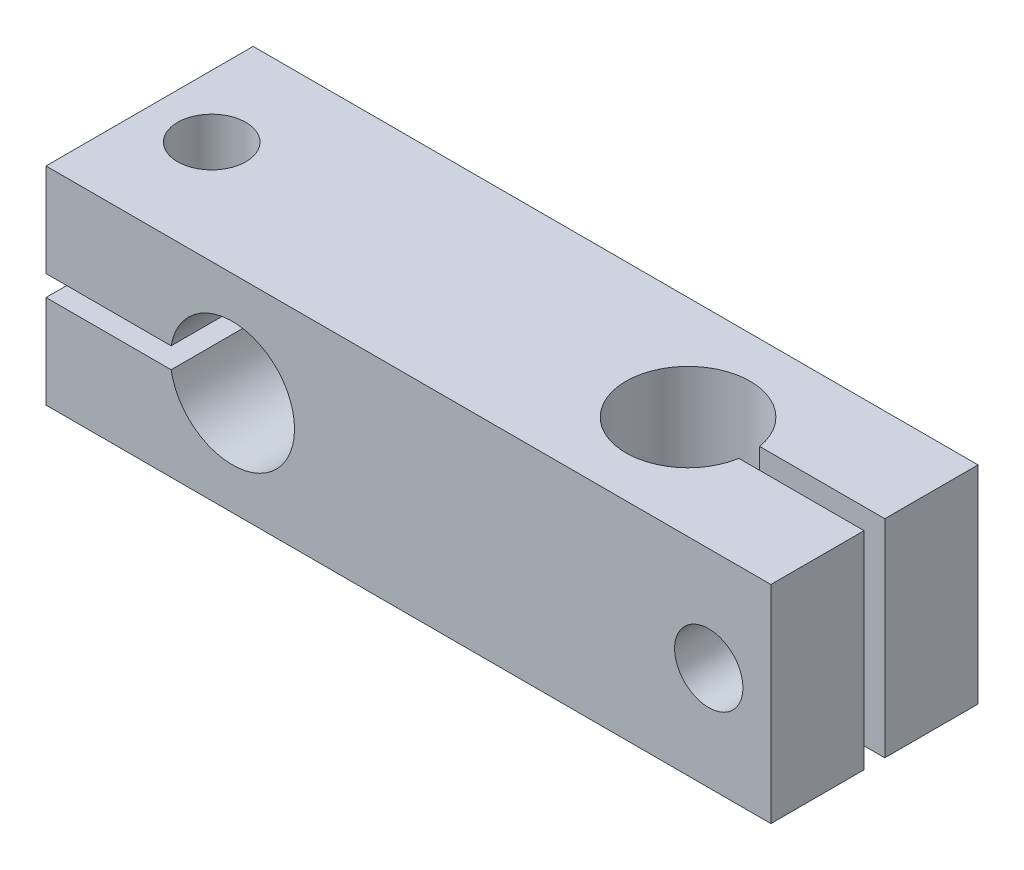
SolidWorks part; units mm, degrees
material "Q235-A"
ref_plane "Front Plane" through (0, 0, 0) normal (0, 0, 1) x (1, 0, 0)
ref_plane "Top Plane" through (0, 0, 0) normal (0, 1, 0) x (1, 0, 0)
ref_plane "Right Plane" through (0, 0, 0) normal (1, 0, 0) x (0, 0, -1)
sketch "Sketch1" plane through (0, 0, 0) normal (0, 0, 1) x (1, 0, 0)
  line L0 (20.5182, 14.6786) -> (28.5182, 14.6786) construction
  line L1 (-41.4818, 24.6786) -> (28.5182, 24.6786)
  line L2 (-41.4818, 24.6786) -> (-41.4818, 15.6786)
  line L3 (-41.4818, 4.6786) -> (28.5182, 4.6786)
  line L4 (28.5182, 24.6786) -> (28.5182, 4.6786)
  line L5 (-41.4818, 13.6786) -> (-41.4818, 4.6786)
  line L6 (-41.4818, 13.6786) -> (-29.3979, 13.6786)
  line L8 (-41.4818, 15.6786) -> (-29.3979, 15.6786)
  arc A0 (-29.3979, 13.6786) -> (-29.3979, 15.6786) centre (-23.4818, 14.6786) ccw
  circle A1 centre (22.5182, 14.6786) radius 2
  dimension "D3" = 12
  dimension "D4" = 18
  dimension "D5" = 46
  dimension "D1" = 70
  dimension "D2" = 20
extrude "Boss-Extrude1" add sketch "Sketch1" along normal blind 20
hole_wizard "Hole1" positions "Sketch2" profile "Sketch3" legacy
sketch "Sketch2" plane through (0, 0, 20) normal (0, 0, 1) x (1, 0, 0)
  point P0 (22.5182, 14.6786)
sketch "Sketch3" plane through (22.5182, 14.6786, 20) normal (1, 0, 0) x (0, -1, 0)
  line L0 (0, 0) -> (0, 9)
  line L1 (0, 9) -> (3.3, 9)
  line L2 (3.3, 9) -> (3.3, 0)
  line L3 (3.3, 0) -> (0, 0)
  line L4 (0, 110) -> (0, -10) construction
  dimension "直径" = 6.6
  dimension "深度" = 9
hole_wizard "M6 Tapped Hole1" positions "Sketch4" profile "Sketch5" tap size "M6" standard "GB"
sketch "Sketch4" plane through (0, 0, 0) normal (0, 0, -1) x (-1, 0, 0)
  point P0 (-22.5182, 14.6786)
sketch "Sketch5" plane through (22.5182, 14.6786, 0) normal (1, 0, 0) x (0, 1, 0)
  line L0 (0, 0) -> (0, 10.5022)
  line L1 (0, 10.5022) -> (2.5, 9)
  line L2 (2.5, 9) -> (2.5, 0)
  line L5 (2.5, 0) -> (0, 0)
  line L10 (0, 10.5022) -> (-2.5, 9) construction
  line L11 (0, -6.35) -> (0, 107.95) construction
  dimension "螺纹孔钻头直径" = 5
  dimension "螺纹孔钻头深度" = 9
  dimension "导头角度" = 118
cosmetic thread "Cosmetic thread 1"
sketch "Sketch6" plane through (0, 24.6786, 0) normal (0, 1, 0) x (1, 0, 0)
  line L0 (-41.4818, -10) -> (28.5182, -10) construction
  line L1 (-41.4818, -20) -> (-41.4818, 0) construction
  line L2 (28.5182, -20) -> (28.5182, 0) construction
  line L4 (16.4343, -11) -> (30.6507, -11)
  line L6 (16.4343, -9) -> (30.6507, -9)
  line L7 (30.6507, -11) -> (30.6507, -9)
  arc A0 (16.4343, -9) -> (16.4343, -11) centre (10.5182, -10) ccw
  circle A1 centre (-35.4818, -10) radius 2
  point P8 (21.5241, -10)
  dimension "D1" = 52
  dimension "D3" = 6
  dimension "D2" = 2
extrude "Cut-Extrude1" cut sketch "Sketch6" against normal through all
hole_wizard "M6 Tapped Hole2" positions "Sketch7" profile "Sketch8" tap size "M6" standard "GB"
sketch "Sketch7" plane through (0, 4.6786, 0) normal (0, -1, 0) x (-1, 0, 0)
  point P0 (35.4818, -10)
sketch "Sketch8" plane through (-35.4818, 4.6786, 10) normal (1, 0, 0) x (0, 0, -1)
  line L0 (0, 0) -> (0, 10.5022)
  line L1 (0, 10.5022) -> (2.5, 9)
  line L2 (2.5, 9) -> (2.5, 0)
  line L5 (2.5, 0) -> (0, 0)
  line L10 (0, 10.5022) -> (-2.5, 9) construction
  line L11 (0, -6.35) -> (0, 107.95) construction
  dimension "螺纹孔钻头直径" = 5
  dimension "螺纹孔钻头深度" = 9
  dimension "导头角度" = 118
cosmetic thread "Cosmetic thread 2"
hole_wizard "Hole2" positions "Sketch9" profile "Sketch10" legacy
sketch "Sketch9" plane through (0, 24.6786, 0) normal (0, 1, 0) x (1, 0, 0)
  point P2 (-35.4818, -10)
sketch "Sketch10" plane through (-35.4818, 24.6786, 10) normal (1, 0, 0) x (0, 0, 1)
  line L0 (0, 0) -> (0, 9)
  line L1 (0, 9) -> (3.3, 9)
  line L2 (3.3, 9) -> (3.3, 0)
  line L3 (3.3, 0) -> (0, 0)
  line L4 (0, 110) -> (0, -10) construction
  dimension "直径" = 6.6
  dimension "深度" = 9
